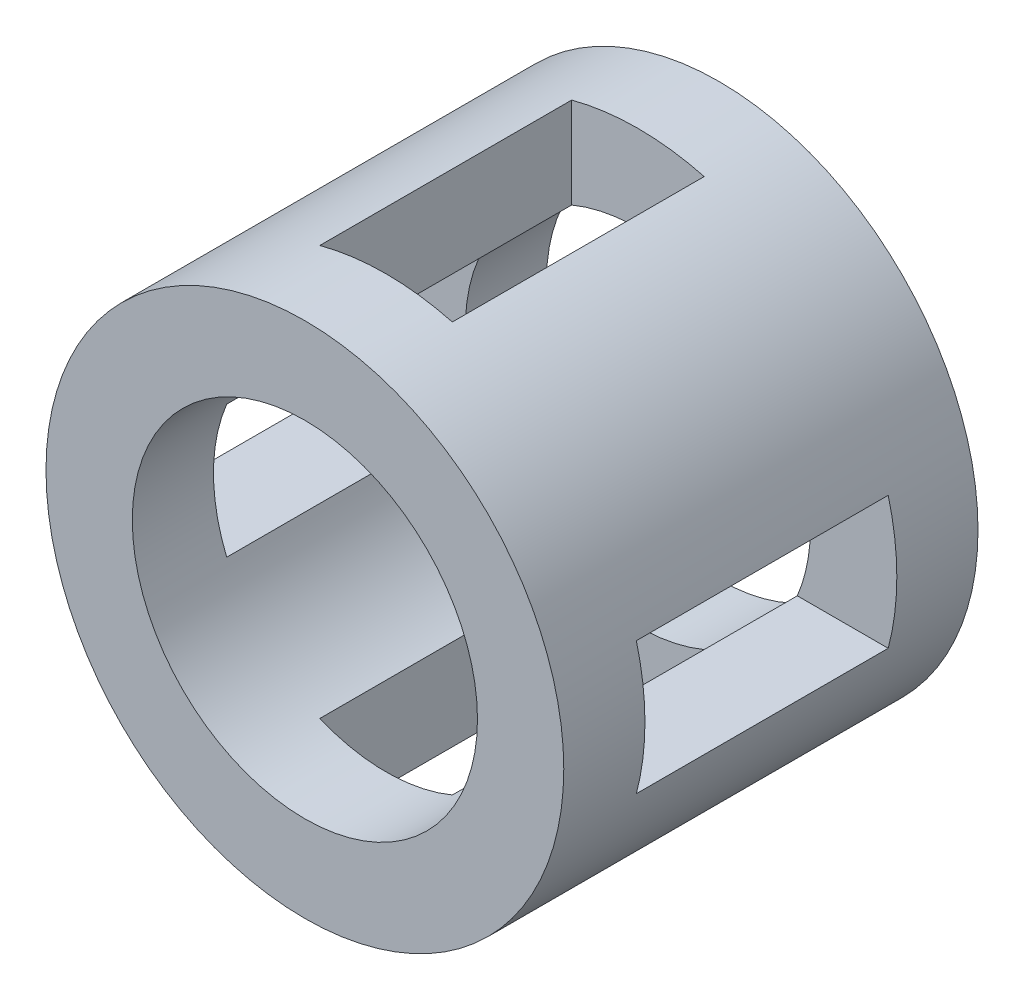
from build123d import *

# Parameters (mm, degrees)
SKETCH1_R           = 75
SKETCH1_R_2         = 50
BOSS_EXTRUDE1_DEPTH = 120
SKETCH2_W           = 38.391183042
SKETCH2_H           = 72.968672404
CUT_EXTRUDE1_DEPTH  = 161.15617378
CIRPATTERN1_COUNT   = 4


with BuildPart() as part:
    # Sketch1 → Boss-Extrude1 (new body)
    with BuildSketch(Plane.XY):
        Circle(SKETCH1_R)
        Circle(SKETCH1_R_2, mode=Mode.SUBTRACT)
    extrude(amount=BOSS_EXTRUDE1_DEPTH)

    # Sketch2 → Cut-Extrude1 (cut, through all)
    with BuildSketch(Plane(origin=(0, 0, 0), x_dir=(1, 0, 0), z_dir=(0, 1, 0))):
        with Locations((0, -60)):
            Rectangle(SKETCH2_W, SKETCH2_H)
    cut_extrude1 = extrude(amount=-CUT_EXTRUDE1_DEPTH, mode=Mode.SUBTRACT)

    # CirPattern1: Cut-Extrude1 ×4 about axis
    cirpattern1_axis = Axis((0, 0, 0), (0, 0, 1))
    for i in range(1, CIRPATTERN1_COUNT):
        add(cut_extrude1.rotate(cirpattern1_axis, i * 360 / CIRPATTERN1_COUNT), mode=Mode.SUBTRACT)


solid = part.part
